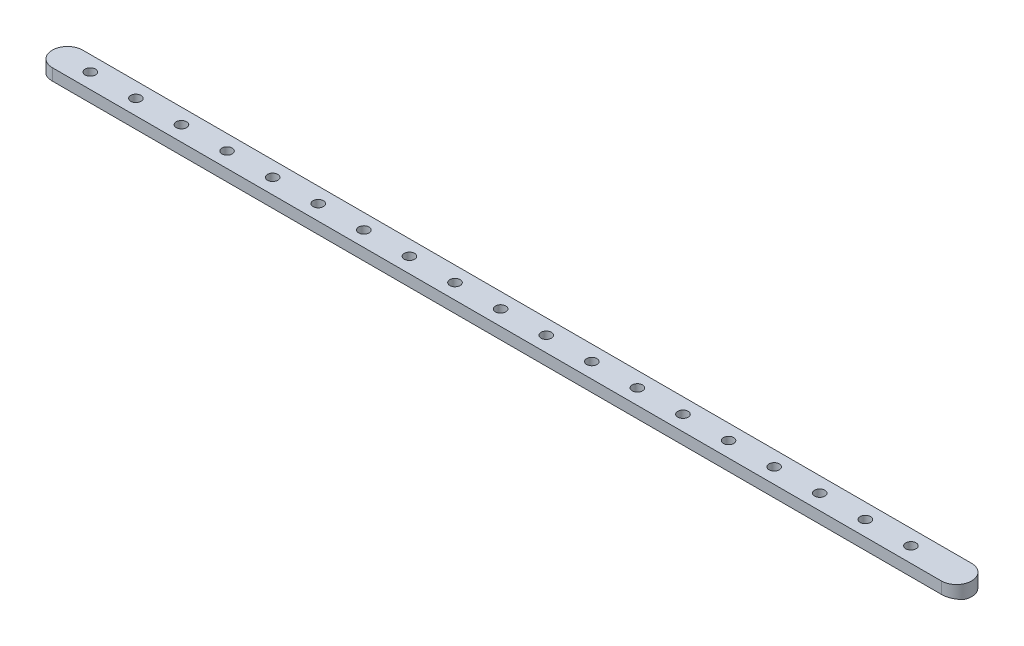
SolidWorks part; units mm, degrees
material "黄铜"
ref_plane "Front Plane" through (0, 0, 0) normal (0, 0, 1) x (1, 0, 0)
ref_plane "Top Plane" through (0, 0, 0) normal (0, 1, 0) x (1, 0, 0)
ref_plane "Right Plane" through (0, 0, 0) normal (1, 0, 0) x (0, 0, -1)
sketch "Sketch1" plane through (0, 0, 0) normal (0, 1, 0) x (1, 0, 0)
  line L0 (-90.9767, 0) -> (494.0233, 0) construction
  line L1 (-90.9767, 10) -> (494.0233, 10)
  line L2 (-90.9767, -10) -> (494.0233, -10)
  arc A0 (-90.9767, 10) -> (-90.9767, -10) centre (-90.9767, 0) ccw
  arc A1 (494.0233, -10) -> (494.0233, 10) centre (494.0233, 0) ccw
  point P2 (201.5233, 0)
  dimension "D2" = 10
  dimension "D1" = 585
extrude "Boss-Extrude1" add sketch "Sketch1" along normal blind 9
hole_wizard "M8 Tapped Hole1" positions "Sketch3" profile "Sketch2" tap size "M8" standard "GB" end condition through all
sketch "Sketch3" plane through (0, 9, 0) normal (0, 1, 0) x (1, 0, 0)
  line L0 (-90.9767, 0) -> (494.0233, 0) construction
  arc A1 (494.0233, -10) -> (494.0233, 10) centre (494.0233, 0) ccw construction
  arc A2 (-90.9767, 10) -> (-90.9767, -10) centre (-90.9767, 0) ccw construction
  point P0 (-75.9767, 0)
  dimension "D1" = 15
sketch "Sketch2" plane through (-75.9767, 9, 0) normal (1, 0, 0) x (0, 0, 1)
  line L0 (0, 0) -> (0, 9)
  line L1 (0, 9) -> (3.4, 9)
  line L2 (3.4, 9) -> (3.4, 0)
  line L5 (3.4, 0) -> (0, 0)
  line L11 (0, -6.35) -> (0, 107.95) construction
  dimension "通孔螺纹孔钻头直径" = 6.8
  dimension "通孔螺纹孔钻头深度" = 9
cosmetic thread "Cosmetic Thread1" parameters "D2"=8
pattern_linear "LPattern1" count 19 spacing 30 along (1, 0, 0) of "M8 Tapped Hole1"
chamfer "Chamfer1" [suppressed] distance 0.5 angle 45
sketch "Sketch4" plane through (0, 0, 0) normal (1, 0, 0) x (0, 0, -1)
  line L0 (0, -6.7552) -> (0, 14.8984) construction
  line L1 (4, -6.7552) -> (4, 16.4542) construction
  line L2 (4, 0) -> (14, 0)
  line L4 (4, 0) -> (14, 2.2169)
  line L5 (14, 2.2169) -> (14, 0)
  line L6 (-14, 2.2169) -> (-14, 0)
  line L7 (-4, 0) -> (-14, 0)
  line L8 (-4, 0) -> (-14, 2.2169)
  dimension "D1" = 4
  dimension "D2" = 12.5
  dimension "D3" = 10
extrude "Cut-Extrude1" cut sketch "Sketch4" along normal through all from offset 200
